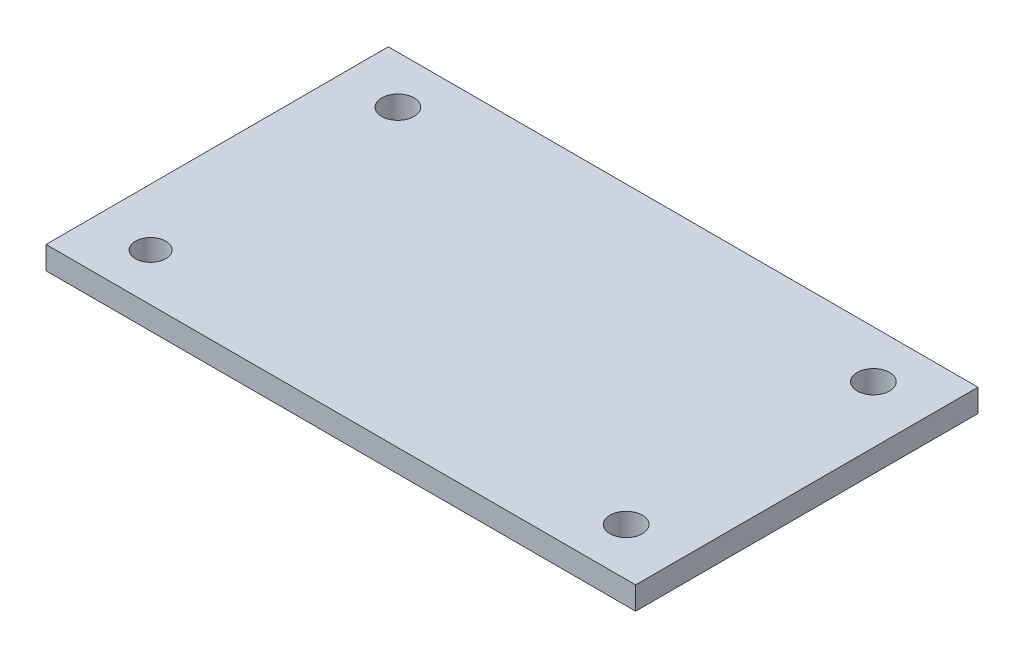
SolidWorks part; units mm, degrees
material "普通碳钢"
ref_plane "Front Plane" through (0, 0, 0) normal (0, 0, 1) x (1, 0, 0)
ref_plane "Top Plane" through (0, 0, 0) normal (0, 1, 0) x (1, 0, 0)
ref_plane "Right Plane" through (0, 0, 0) normal (1, 0, 0) x (0, 0, -1)
sketch "Sketch1" plane through (0, 0, 0) normal (0, 1, 0) x (1, 0, 0)
  line L0 (-125, 65) -> (125, 65) construction
  line L1 (-125, 65) -> (-125, -65) construction
  line L2 (-155, 90) -> (155, 90)
  line L3 (155, 90) -> (155, -90)
  line L4 (155, -90) -> (-155, -90)
  line L5 (-155, -90) -> (-155, 90)
  circle A0 centre (125, -65) radius 8.5
  circle A1 centre (-125, -65) radius 8
  circle A2 centre (-125, 65) radius 8.5
  circle A3 centre (125, 65) radius 8.5
  point P8 (0, 65)
  point P9 (-125, 0)
  dimension "D1" = 17
  dimension "D2" = 17
  dimension "D3" = 17
  dimension "D4" = 16
  dimension "D5" = 250
  dimension "D6" = 130
  dimension "D7" = 250
  dimension "D8" = 180
  dimension "D9" = 310
  dimension "D10" = 155
  dimension "D11" = 25
extrude "Extrude1" add sketch "Sketch1" along normal mid plane 12
